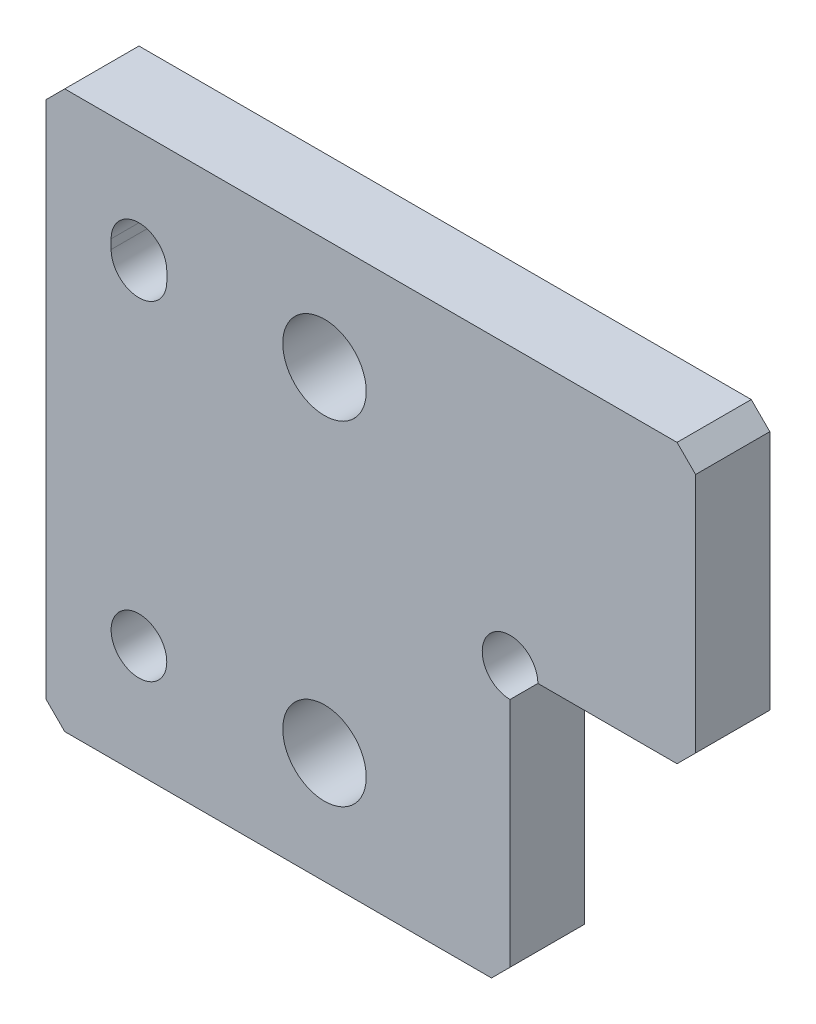
from build123d import *

# Parameters (mm, degrees)
SKETCH1_W                  = 35
SKETCH1_H                  = 30
BOSS_EXTRUDE1_DEPTH        = 2
SKETCH2_W                  = 10
SKETCH2_H                  = 15
CUT_EXTRUDE1_DEPTH         = 24.393375131
F_3_0_3_DIAMETER_HOLE2_D   = 3
F_3_0_3_DIAMETER_HOLE1_D   = 3
F_4_5_4_5_DIAMETER_HOLE1_D = 4.5
CHAMFER1_SIZE              = 1
CUT_EXTRUDE2_DEPTH         = 24.393375131


with BuildPart() as part:
    # Sketch1 → Boss-Extrude1 (new, symmetric)
    with BuildSketch(Plane.XY):
        Rectangle(SKETCH1_W, SKETCH1_H)
    extrude(amount=BOSS_EXTRUDE1_DEPTH, both=True)

    # Sketch2 → Cut-Extrude1 (cut, through all)
    with BuildSketch(Plane.XY.offset(2)):
        with Locations((12.5, -7.5)):
            Rectangle(SKETCH2_W, SKETCH2_H)
    extrude(amount=-CUT_EXTRUDE1_DEPTH, mode=Mode.SUBTRACT)

    # Ø3.0 (3) Diameter Hole2 (through all)
    with Locations(Plane.XY.offset(2)):
        with Locations((7.5, 0)):
            Hole(F_3_0_3_DIAMETER_HOLE2_D / 2)

    # Ø3.0 (3) Diameter Hole1 (through all)
    with Locations(Plane.XY.offset(2)):
        with Locations((-12.5, 9), (-12.5, -9)):
            Hole(F_3_0_3_DIAMETER_HOLE1_D / 2)

    # Ø4.5 (4.5) Diameter Hole1 (through all)
    with Locations(Plane.XY.offset(2)):
        with Locations((-2.5, 9), (-2.5, -9)):
            Hole(F_4_5_4_5_DIAMETER_HOLE1_D / 2)

    # Chamfer1
    chamfer1_edges = [part.edges().sort_by_distance(p)[0] for p in [
        (17.5, 0, 0),
        (7.5, -15, 0),
        (-17.5, -15, 0),
        (-17.5, 15, 0),
        (17.5, 15, 0),
    ]]
    chamfer(chamfer1_edges, length=CHAMFER1_SIZE)

    # Sketch9 → Cut-Extrude2 (cut, through all)
    with BuildSketch(Plane.XY.offset(2)):
        with BuildLine():
            Line((-11, 9.25), (-11, 8.75))
            ThreePointArc((-11, 8.75), (-12.5, 7.25), (-14, 8.75))
            Line((-14, 8.75), (-14, 9.25))
            ThreePointArc((-14, 9.25), (-12.5, 10.75), (-11, 9.25))
        make_face()
    extrude(amount=-CUT_EXTRUDE2_DEPTH, mode=Mode.SUBTRACT)


solid = part.part
